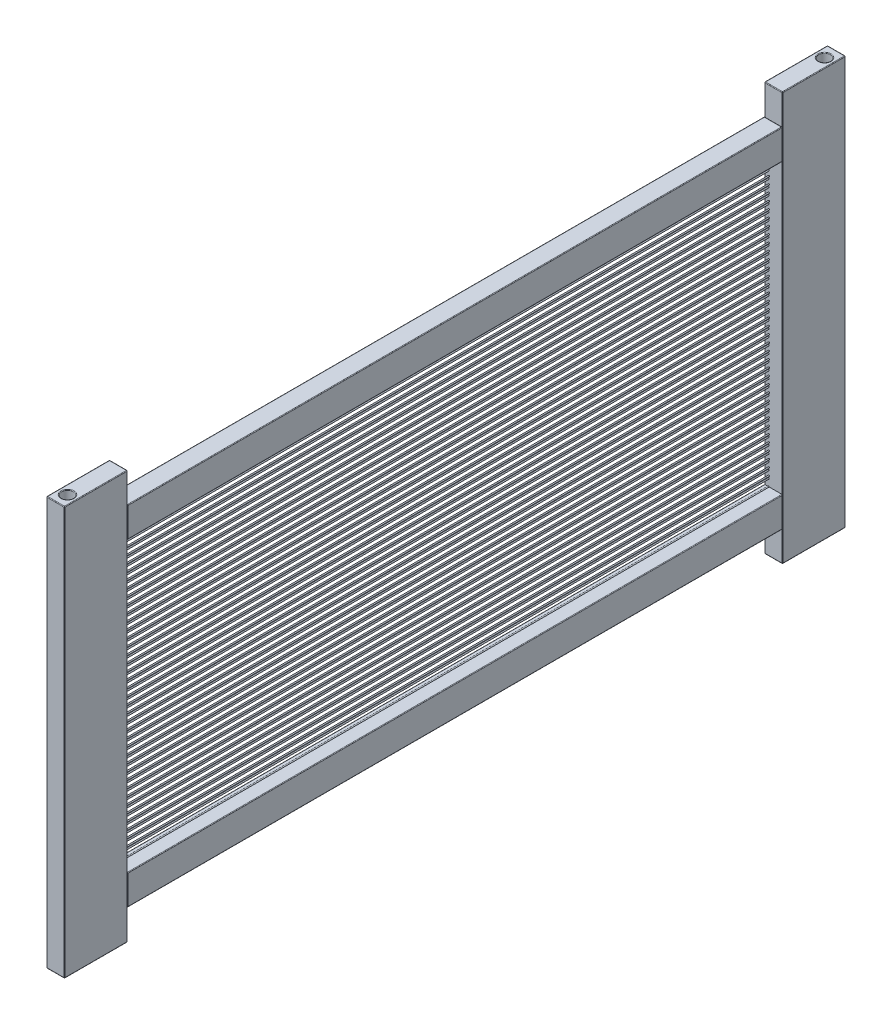
SolidWorks part; units mm, degrees
ref_plane "Front" through (0, 0, 0) normal (0, 0, 1) x (1, 0, 0)
ref_plane "Top" through (0, 0, 0) normal (0, 1, 0) x (1, 0, 0)
ref_plane "Right" through (0, 0, 0) normal (1, 0, 0) x (0, 0, -1)
sketch "草图1" plane through (0, 0, 0) normal (0, 1, 0) x (1, 0, 0)
  line L1 (-15, -52.5) -> (15, -52.5)
  line L2 (-15, -52.5) -> (-15, 52.5)
  line L3 (-15, 52.5) -> (15, 52.5)
  line L4 (15, -52.5) -> (15, 52.5)
  line L5 (-15, -52.5) -> (15, 52.5) construction
  line L6 (-15, 52.5) -> (15, -52.5) construction
  line L7 (-15, 1247.5) -> (15, 1247.5)
  line L8 (-15, 1247.5) -> (-15, 1142.5)
  line L9 (-15, 1142.5) -> (15, 1142.5)
  line L10 (15, 1247.5) -> (15, 1142.5)
  line L11 (-15, 1247.5) -> (15, 1142.5) construction
  line L12 (-15, 1142.5) -> (15, 1247.5) construction
  point P0 (0, 0)
  point P6 (0, 1195)
  dimension "D1" = 30
  dimension "D2" = 105
  dimension "D3" = 30
  dimension "D4" = 105
  dimension "D5" = 0
  dimension "D6" = 1300
extrude "凸台-拉伸1" add sketch "草图1" along normal blind 680
sketch "草图2" plane through (0, 0, 0) normal (0, -1, 0) x (1, 0, 0)
  line L0 (-15, 52.5) -> (15, 52.5) construction
  line L1 (15, -1142.5) -> (15, -1247.5) construction
  line L2 (15, -1247.5) -> (-15, -1247.5) construction
  circle A0 centre (0, 32.5) radius 10
  circle A1 centre (0, -1227.5) radius 10
  dimension "D1" = 20
  dimension "D2" = 20
  dimension "D3" = 20
  dimension "D4" = 15
  dimension "D5" = 20
extrude "切除-拉伸1" cut sketch "草图2" against normal through all
sketch "草图6" plane through (0, 0, -1142.5) normal (0, 0, 1) x (1, 0, 0)
  line L0 (-15, 680) -> (-15, 0) construction
  line L1 (-15, 50) -> (15, 50)
  line L2 (-15, 50) -> (-15, 100)
  line L3 (-15, 100) -> (15, 100)
  line L4 (15, 50) -> (15, 100)
  line L5 (15, 680) -> (15, 0) construction
  line L6 (-15, 680) -> (15, 680) construction
  line L7 (-15, 630) -> (15, 630)
  line L8 (-15, 630) -> (-15, 580)
  line L9 (-15, 580) -> (15, 580)
  line L10 (15, 630) -> (15, 580)
  line L11 (-15, 0) -> (15, 0) construction
  dimension "D1" = 50
  dimension "D2" = 50
  dimension "D3" = 50
  dimension "D4" = 50
extrude "凸台-拉伸2" add sketch "草图6" along normal up to surface (1090 mm away) separate body up to face at (0, 340, -52.5)
sketch "草图7" plane through (0, 0, -1142.5) normal (0, 0, 1) x (1, 0, 0)
  line L0 (-15, 0) -> (15, 0) construction
  circle A0 centre (-8, 568) radius 1
  circle A1 centre (-7.5511, 583.9937) radius 1
  circle A2 centre (-8, 556) radius 1
  circle A3 centre (-7.5511, 571.9937) radius 1
  circle A4 centre (-8, 544) radius 1
  circle A5 centre (-7.5511, 559.9937) radius 1
  circle A6 centre (-8, 532) radius 1
  circle A7 centre (-7.5511, 547.9937) radius 1
  circle A8 centre (-8, 520) radius 1
  circle A9 centre (-7.5511, 535.9937) radius 1
  circle A10 centre (-8, 508) radius 1
  circle A11 centre (-7.5511, 523.9937) radius 1
  circle A12 centre (-8, 496) radius 1
  circle A13 centre (-7.5511, 511.9937) radius 1
  circle A14 centre (-8, 484) radius 1
  circle A15 centre (-7.5511, 499.9937) radius 1
  circle A16 centre (-8, 472) radius 1
  circle A17 centre (-7.5511, 487.9937) radius 1
  circle A18 centre (-8, 460) radius 1
  circle A19 centre (-7.5511, 475.9937) radius 1
  circle A20 centre (-8, 448) radius 1
  circle A21 centre (-7.5511, 463.9937) radius 1
  circle A22 centre (-8, 436) radius 1
  circle A23 centre (-7.5511, 451.9937) radius 1
  circle A24 centre (-8, 424) radius 1
  circle A25 centre (-7.5511, 439.9937) radius 1
  circle A26 centre (-8, 412) radius 1
  circle A27 centre (-7.5511, 427.9937) radius 1
  circle A28 centre (-8, 400) radius 1
  circle A29 centre (-7.5511, 415.9937) radius 1
  circle A30 centre (-8, 388) radius 1
  circle A31 centre (-7.5511, 403.9937) radius 1
  circle A32 centre (-8, 376) radius 1
  circle A33 centre (-7.5511, 391.9937) radius 1
  circle A34 centre (-8, 364) radius 1
  circle A35 centre (-7.5511, 379.9937) radius 1
  circle A36 centre (-8, 352) radius 1
  circle A37 centre (-7.5511, 367.9937) radius 1
  circle A38 centre (-8, 340) radius 1
  circle A39 centre (-7.5511, 355.9937) radius 1
  circle A40 centre (-8, 328) radius 1
  circle A41 centre (-7.5511, 343.9937) radius 1
  circle A42 centre (-8, 316) radius 1
  circle A43 centre (-7.5511, 331.9937) radius 1
  circle A44 centre (-8, 304) radius 1
  circle A45 centre (-7.5511, 319.9937) radius 1
  circle A46 centre (-8, 292) radius 1
  circle A47 centre (-7.5511, 307.9937) radius 1
  circle A48 centre (-8, 280) radius 1
  circle A49 centre (-7.5511, 295.9937) radius 1
  circle A50 centre (-8, 268) radius 1
  circle A51 centre (-7.5511, 283.9937) radius 1
  circle A52 centre (-8, 256) radius 1
  circle A53 centre (-7.5511, 271.9937) radius 1
  circle A54 centre (-8, 244) radius 1
  circle A55 centre (-7.5511, 259.9937) radius 1
  circle A56 centre (-8, 232) radius 1
  circle A57 centre (-7.5511, 247.9937) radius 1
  circle A58 centre (-8, 220) radius 1
  circle A59 centre (-7.5511, 235.9937) radius 1
  circle A60 centre (-8, 208) radius 1
  circle A61 centre (-7.5511, 223.9937) radius 1
  circle A62 centre (-8, 196) radius 1
  circle A63 centre (-7.5511, 211.9937) radius 1
  circle A64 centre (-8, 184) radius 1
  circle A65 centre (-7.5511, 199.9937) radius 1
  circle A66 centre (-8, 172) radius 1
  circle A67 centre (-7.5511, 187.9937) radius 1
  circle A68 centre (-8, 160) radius 1
  circle A69 centre (-7.5511, 175.9937) radius 1
  circle A70 centre (-8, 148) radius 1
  circle A71 centre (-7.5511, 163.9937) radius 1
  circle A72 centre (-8, 136) radius 1
  circle A73 centre (-7.5511, 151.9937) radius 1
  circle A74 centre (-8, 124) radius 1
  circle A75 centre (-7.5511, 139.9937) radius 1
  circle A76 centre (-8, 112) radius 1
  circle A77 centre (-7.5511, 127.9937) radius 1
  circle A78 centre (-8, 100) radius 1
  circle A79 centre (-7.5511, 115.9937) radius 1
  point P6 (0, 0)
  dimension "D1" = 16
  dimension "D2" = 8
  dimension "D3" = 2
  dimension "D4" = 12
  dimension "D5" = 40
extrude "凸台-拉伸3" add sketch "草图7" along normal up to surface (1090 mm away) separate body up to face at (0, 340, -52.5)
fillet "圆角1" radius 1 14 edges at (0, 680, -52.5) (0, 680, 22.5) (15, 680, 0) (15, 340, -52.5) (0, 0, -52.5) (15, 0, 0) (0, 0, 22.5) (0, 680, 52.5) (15, 340, 52.5) (0, 0, 52.5) (-15, 340, -52.5) (-15, 680, 0) (-15, 340, 52.5) (-15, 0, 0)
fillet "圆角2" radius 1 10 edges at (-15, 580, -597.5) (-15, 605, -1142.5) (-15, 605, -52.5) (15, 605, -1142.5) (15, 580, -597.5) (15, 605, -52.5) (-15, 630, -597.5) (0, 630, -1142.5) (15, 630, -597.5) (0, 630, -52.5)
fillet "圆角3" radius 1 13 edges at (0, 0, -1247.5) (15, 340, -1247.5) (15, 0, -1195) (0, 680, -1247.5) (15, 680, -1195) (0, 680, -1237.5) (0, 680, -1142.5) (15, 340, -1142.5) (0, 0, -1142.5) (-15, 340, -1247.5) (-15, 680, -1195) (-15, 340, -1142.5) (-15, 0, -1195)
fillet "圆角4" radius 1 10 edges at (-15, 75, -1142.5) (-15, 100, -597.5) (-15, 75, -52.5) (0, 50, -1142.5) (-15, 50, -597.5) (0, 50, -52.5) (15, 100, -597.5) (15, 75, -1142.5) (15, 50, -597.5) (15, 75, -52.5)
